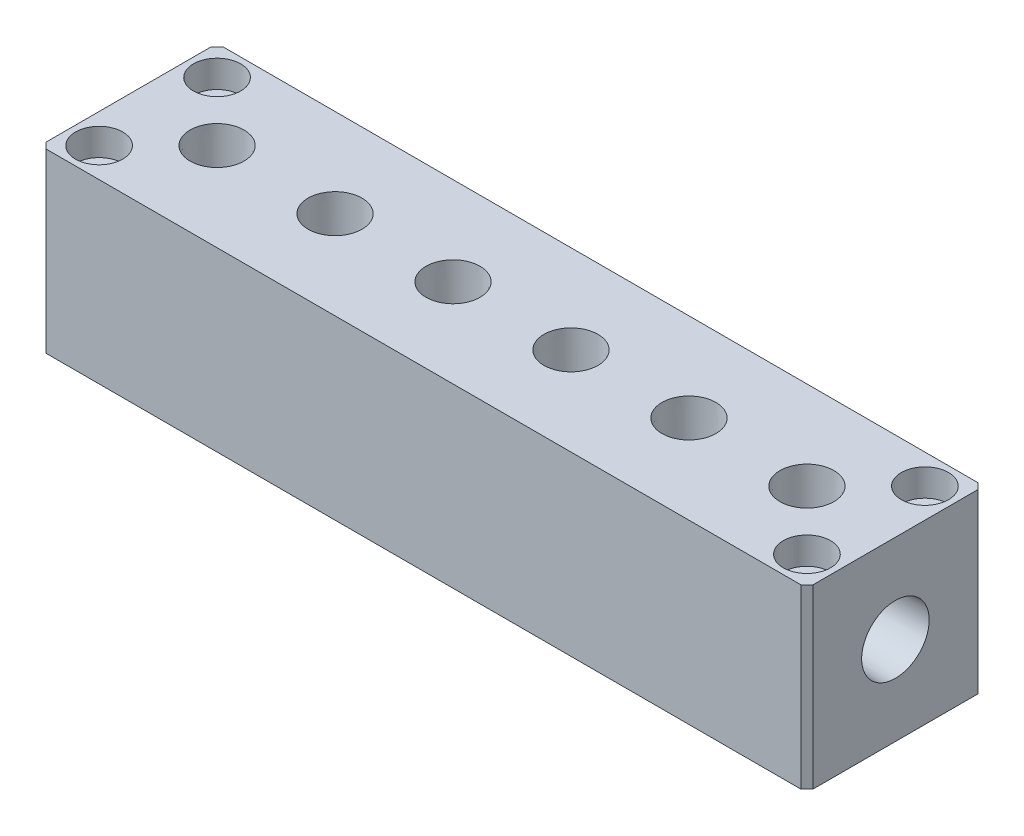
SolidWorks part; units mm, degrees
material "A6061"
ref_plane "前基準面" through (0, 0, 0) normal (0, 0, 1) x (1, 0, 0)
ref_plane "上基準面" through (0, 0, 0) normal (0, 1, 0) x (1, 0, 0)
ref_plane "右基準面" through (0, 0, 0) normal (1, 0, 0) x (0, 0, -1)
sketch "草图1" plane through (0, 0, 0) normal (0, 1, 0) x (1, 0, 0)
  line L1 (-65, -15) -> (65, -15)
  line L2 (-65, -15) -> (-65, 15)
  line L3 (-65, 15) -> (65, 15)
  line L4 (65, -15) -> (65, 15)
  line L5 (-65, -15) -> (65, 15) construction
  line L6 (-65, 15) -> (65, -15) construction
  point P0 (0, 0)
  dimension "D1" = 130
  dimension "D2" = 30
extrude "凸台-拉伸1" add sketch "草图1" along normal mid plane 30
hole_wizard "1/4 Rc 螺纹孔1" positions "草图2" profile "草图4" size "1/4" standard "GB"
sketch "草图2" plane through (65, 0, 0) normal (1, 0, 0) x (0, 0, -1)
  point P0 (0, 0)
sketch "草图4" plane through (65, 0, 0) normal (0, 1, 0) x (0, 0, -1)
  line L0 (0, 0) -> (0, 123.2146)
  line L1 (5.35, 120) -> (0, 123.2146)
  line L2 (-5.35, 120) -> (0, 123.2146) construction
  line L3 (5.35, 120) -> (5.35, 11)
  line L4 (5.35, 11) -> (5.3791, 11)
  line L5 (5.3791, 11) -> (5.7225, 0)
  line L6 (-5.3791, 11) -> (-5.7225, 0) construction
  line L7 (5.7225, 0) -> (0, 0)
  line L8 (0, -6.35) -> (0, 107.95) construction
  line L11 (-5.35, 11) -> (-5.3791, 11) construction
  dimension "螺纹孔钻头直径" = 10.7
  dimension "螺纹孔钻头深度" = 120
  dimension "螺纹直径" = 11.445
  dimension "螺纹角度" = 3.576
  dimension "螺纹深度" = 11
  dimension "导头角度" = 118
hole_wizard "1/8 Rc 螺纹孔1" positions "草图7" profile "草图8" size "1/8" standard "GB"
sketch "草图7" plane through (0, 15, 0) normal (0, 1, 0) x (1, 0, 0)
  line L0 (0, 0) -> (0, 19.2628) construction
  point P0 (50, 0)
  point P5 (30, 0)
  point P6 (10, 0)
  point P7 (-10, 0)
  point P8 (-30, 0)
  point P9 (-50, 0)
  dimension "D2" = 20
  dimension "D1" = 6
sketch "草图8" plane through (50, 15, 0) normal (1, 0, 0) x (0, 0, 1)
  line L0 (0, 0) -> (0, 14.3134)
  line L1 (3.95, 11.94) -> (0, 14.3134)
  line L2 (-3.95, 11.94) -> (0, 14.3134) construction
  line L3 (3.95, 11.94) -> (3.95, 7.4)
  line L4 (3.95, 7.4) -> (4.3425, 7.4)
  line L5 (4.3425, 7.4) -> (4.5735, 0)
  line L6 (-4.3425, 7.4) -> (-4.5735, 0) construction
  line L7 (4.5735, 0) -> (0, 0)
  line L8 (0, -6.35) -> (0, 107.95) construction
  line L11 (-3.95, 7.4) -> (-4.3425, 7.4) construction
  dimension "螺纹孔钻头直径" = 7.9
  dimension "螺纹孔钻头深度" = 11.94
  dimension "螺纹直径" = 9.147
  dimension "螺纹角度" = 3.576
  dimension "螺纹深度" = 7.4
  dimension "导头角度" = 118
cosmetic thread "孔螺蚊线1"
cosmetic thread "孔螺蚊线2"
cosmetic thread "孔螺蚊线3"
cosmetic thread "孔螺蚊线4"
cosmetic thread "孔螺蚊线5"
cosmetic thread "孔螺蚊线6"
chamfer "倒角1" distance 1 angle 45 4 edges at (65, 0, -15) (65, 0, 15) (-65, 0, 15) (-65, 0, -15)
hole_wizard "打孔尺寸(%根据)内六角圆柱头螺钉的类型1" positions "草图9" profile "草图10" counterbore size "M4" standard "GB" end condition through all
sketch "草图9" plane through (0, 15, 0) normal (0, 1, 0) x (1, 0, 0)
  line L0 (0, 25.1955) -> (0, 0) construction
  line L1 (0, 0) -> (-67.1651, 0) construction
  line L3 (64, 15) -> (-64, 15) construction
  point P0 (-60, 10)
  point P10 (-60, -10)
  point P11 (60, -10)
  point P12 (60, 10)
  dimension "D1" = 120
  dimension "D2" = 5
sketch "草图10" plane through (-60, 15, -10) normal (1, 0, 0) x (0, 0, 1)
  line L0 (0, 0) -> (0, 30)
  line L1 (0, 30) -> (2.25, 30)
  line L3 (2.25, 30) -> (2.25, 4.6)
  line L4 (2.25, 4.6) -> (4, 4.6)
  line L5 (4, 4.6) -> (4, 0)
  line L7 (4, 0) -> (0, 0)
  line L11 (0, -6.35) -> (0, 107.95) construction
  dimension "通孔孔直径" = 4.5
  dimension "通孔孔深度" = 30
  dimension "柱形沉头孔直径" = 8
  dimension "柱形沉头孔深度" = 4.6
